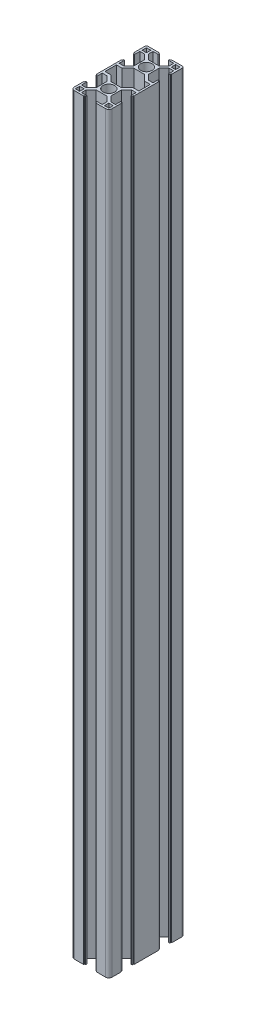
from build123d import *

# Parameters (mm, degrees)
SKETCH1_R                                = 4.6
SKETCH1_W                                = 3.5
SKETCH1_H                                = 3.5
ALUMINUM_PROFILE_30_X_60L_X_R2_5_1_DEPTH = 600


with BuildPart() as part:
    # Sketch1 → Aluminum profile 30 X 60L X R2.5(1) (new body)
    with BuildSketch(Plane(origin=(0, 0, 0), x_dir=(-1, 0, 0), z_dir=(0, 1, 0))):
        with BuildLine():
            Line((-5.1, 15), (-5.1, 14.5))
            Line((-5.1, 14.5), (-4.1, 14.5))
            Line((-4.1, 14.5), (-4.1, 13.5))
            Line((-4.1, 13.5), (-8.25, 13.5))
            Line((-8.25, 13.5), (-8.25, 9.8))
            Line((-8.25, 9.8), (-4.25, 5.8))
            Line((-4.25, 5.8), (4.25, 5.8))
            Line((4.25, 5.8), (8.25, 9.8))
            Line((8.25, 9.8), (8.25, 13.5))
            Line((8.25, 13.5), (4.1, 13.5))
            Line((4.1, 13.5), (4.1, 14.5))
            Line((4.1, 14.5), (5.1, 14.5))
            Line((5.1, 14.5), (5.1, 15))
            Line((5.1, 15), (12.5, 15))
            ThreePointArc((12.5, 15), (14.267766953, 14.267766953), (15, 12.5))
            Line((15, 12.5), (15, 5.1))
            Line((15, 5.1), (14.5, 5.1))
            Line((14.5, 5.1), (14.5, 4.1))
            Line((14.5, 4.1), (13.5, 4.1))
            Line((13.5, 4.1), (13.5, 8.25))
            Line((13.5, 8.25), (9.8, 8.25))
            Line((9.8, 8.25), (5.8, 4.25))
            Line((5.8, 4.25), (5.8, -4.25))
            Line((5.8, -4.25), (9.8, -8.25))
            Line((9.8, -8.25), (13.5, -8.25))
            Line((13.5, -8.25), (13.5, -4.1))
            Line((13.5, -4.1), (14.5, -4.1))
            Line((14.5, -4.1), (14.5, -5.1))
            Line((14.5, -5.1), (15, -5.1))
            Line((15, -5.1), (15, -24.9))
            Line((15, -24.9), (14.5, -24.9))
            Line((14.5, -24.9), (14.5, -25.9))
            Line((14.5, -25.9), (13.5, -25.9))
            Line((13.5, -25.9), (13.5, -21.75))
            Line((13.5, -21.75), (9.8, -21.75))
            Line((9.8, -21.75), (5.8, -25.75))
            Line((5.8, -25.75), (5.8, -34.25))
            Line((5.8, -34.25), (9.8, -38.25))
            Line((9.8, -38.25), (13.5, -38.25))
            Line((13.5, -38.25), (13.5, -34.1))
            Line((13.5, -34.1), (14.5, -34.1))
            Line((14.5, -34.1), (14.5, -35.1))
            Line((14.5, -35.1), (15, -35.1))
            Line((15, -35.1), (15, -43.5))
            ThreePointArc((15, -43.5), (14.560660172, -44.560660172), (13.5, -45))
            Line((13.5, -45), (5.1, -45))
            Line((5.1, -45), (5.1, -44.5))
            Line((5.1, -44.5), (4.1, -44.5))
            Line((4.1, -44.5), (4.1, -43.5))
            Line((4.1, -43.5), (8.25, -43.5))
            Line((8.25, -43.5), (8.25, -39.8))
            Line((8.25, -39.8), (4.25, -35.8))
            Line((4.25, -35.8), (-4.25, -35.8))
            Line((-4.25, -35.8), (-8.25, -39.8))
            Line((-8.25, -39.8), (-8.25, -43.5))
            Line((-8.25, -43.5), (-4.1, -43.5))
            Line((-4.1, -43.5), (-4.1, -44.5))
            Line((-4.1, -44.5), (-5.1, -44.5))
            Line((-5.1, -44.5), (-5.1, -45))
            Line((-5.1, -45), (-13.5, -45))
            ThreePointArc((-13.5, -45), (-14.560660172, -44.560660172), (-15, -43.5))
            Line((-15, -43.5), (-15, -35.1))
            Line((-15, -35.1), (-14.5, -35.1))
            Line((-14.5, -35.1), (-14.5, -34.1))
            Line((-14.5, -34.1), (-13.5, -34.1))
            Line((-13.5, -34.1), (-13.5, -38.25))
            Line((-13.5, -38.25), (-9.8, -38.25))
            Line((-9.8, -38.25), (-5.8, -34.25))
            Line((-5.8, -34.25), (-5.8, -25.75))
            Line((-5.8, -25.75), (-9.8, -21.75))
            Line((-9.8, -21.75), (-13.5, -21.75))
            Line((-13.5, -21.75), (-13.5, -25.9))
            Line((-13.5, -25.9), (-14.5, -25.9))
            Line((-14.5, -25.9), (-14.5, -24.9))
            Line((-14.5, -24.9), (-15, -24.9))
            Line((-15, -24.9), (-15, -5.1))
            Line((-15, -5.1), (-14.5, -5.1))
            Line((-14.5, -5.1), (-14.5, -4.1))
            Line((-14.5, -4.1), (-13.5, -4.1))
            Line((-13.5, -4.1), (-13.5, -8.25))
            Line((-13.5, -8.25), (-9.8, -8.25))
            Line((-9.8, -8.25), (-5.8, -4.25))
            Line((-5.8, -4.25), (-5.8, 4.25))
            Line((-5.8, 4.25), (-9.8, 8.25))
            Line((-9.8, 8.25), (-13.5, 8.25))
            Line((-13.5, 8.25), (-13.5, 4.1))
            Line((-13.5, 4.1), (-14.5, 4.1))
            Line((-14.5, 4.1), (-14.5, 5.1))
            Line((-14.5, 5.1), (-15, 5.1))
            Line((-15, 5.1), (-15, 12.5))
            ThreePointArc((-15, 12.5), (-14.267766953, 14.267766953), (-12.5, 15))
            Line((-12.5, 15), (-5.1, 15))
        make_face()
        Circle(SKETCH1_R, mode=Mode.SUBTRACT)
        with Locations((0, -30)):
            Circle(SKETCH1_R, mode=Mode.SUBTRACT)
        Polygon((8.9, -10.45), (4.25, -5.8), (-4.25, -5.8), (-8.9, -10.45), (-13.5, -10.45), (-13.5, -19.55), (-8.9, -19.55), (-4.25, -24.2), (4.25, -24.2), (8.9, -19.55), (13.5, -19.55), (13.5, -10.45), align=None, mode=Mode.SUBTRACT)
        with Locations((-11.625, 11.625)):
            Rectangle(SKETCH1_W, SKETCH1_H, mode=Mode.SUBTRACT)
        with Locations((11.625, 11.625)):
            Rectangle(SKETCH1_W, SKETCH1_H, mode=Mode.SUBTRACT)
        with Locations((-11.625, -41.625)):
            Rectangle(SKETCH1_W, SKETCH1_H, mode=Mode.SUBTRACT)
        with Locations((11.625, -41.625)):
            Rectangle(SKETCH1_W, SKETCH1_H, mode=Mode.SUBTRACT)
    extrude(amount=ALUMINUM_PROFILE_30_X_60L_X_R2_5_1_DEPTH)


solid = part.part
